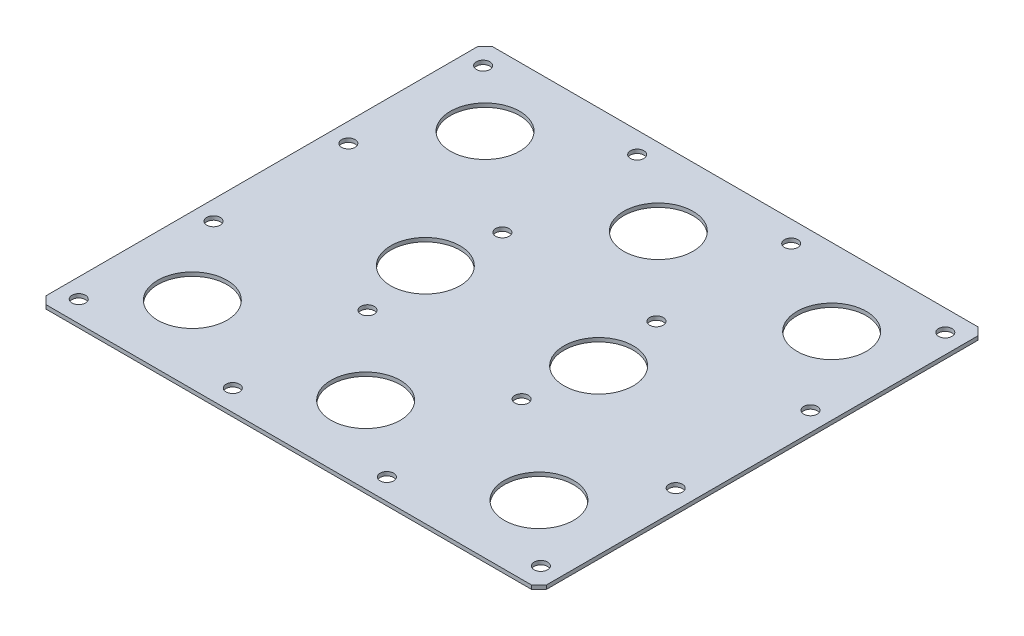
from build123d import *

# Parameters (mm, degrees)
SKETCH1_W                  = 130
SKETCH1_H                  = 116
BOSS_EXTRUDE1_DEPTH        = 1
SKETCH2_R                  = 9
CUT_EXTRUDE1_DEPTH         = 88.120606058
LPATTERN1_COUNT            = 3
LPATTERN1_PITCH            = 38
LPATTERN1_COUNT_DIR2       = 5
LPATTERN1_PITCH_DIR2       = 22.5
CHAMFER1_SIZE              = 2
F_3_5_3_5_DIAMETER_HOLE1_D = 3.5
LPATTERN2_COUNT            = 4
LPATTERN2_PITCH            = 40
LPATTERN2_COUNT_DIR2       = 4
LPATTERN2_PITCH_DIR2       = 35


with BuildPart() as part:
    # Sketch1 → Boss-Extrude1 (new body)
    with BuildSketch(Plane(origin=(0, 0, 0), x_dir=(1, 0, 0), z_dir=(0, 1, 0))):
        Rectangle(SKETCH1_W, SKETCH1_H)
    extrude(amount=BOSS_EXTRUDE1_DEPTH)

    # Sketch2 → Cut-Extrude1 (cut, through all)
    with BuildSketch(Plane(origin=(0, 1, 0), x_dir=(1, 0, 0), z_dir=(0, 1, 0))):
        with Locations(Location((45, -38, 0), (0, 0, 270))):
            Circle(SKETCH2_R)
    cut_extrude1 = extrude(amount=-CUT_EXTRUDE1_DEPTH, mode=Mode.SUBTRACT)

    # LPattern1: Cut-Extrude1 3 × 5, 7 skipped
    with Locations(*[(-j * LPATTERN1_PITCH_DIR2, 0, -i * LPATTERN1_PITCH) for i in range(LPATTERN1_COUNT) for j in range(LPATTERN1_COUNT_DIR2) if (i, j) not in ((0, 0), (0, 1), (0, 3), (1, 0), (1, 2), (1, 4), (2, 1), (2, 3))]):
        add(cut_extrude1, mode=Mode.SUBTRACT)

    # Chamfer1
    chamfer1_edges = [part.edges().sort_by_distance(p)[0] for p in [
        (65, 0.5, 58),
        (-65, 0.5, 58),
        (-65, 0.5, -58),
        (65, 0.5, -58),
    ]]
    chamfer(chamfer1_edges, length=CHAMFER1_SIZE)

    # Ø3.5 (3.5) Diameter Hole1 (through all)
    with Locations(Plane(origin=(0, 1, 0), x_dir=(1, 0, 0), z_dir=(0, 1, 0))):
        with Locations((60, -52.5)):
            f_3_5_3_5_diameter_hole1 = Hole(F_3_5_3_5_DIAMETER_HOLE1_D / 2)

    # LPattern2: 3.5 _3.5_ Diameter Hole1 4 × 4
    with Locations(*[(-i * LPATTERN2_PITCH, 0, -j * LPATTERN2_PITCH_DIR2) for i in range(LPATTERN2_COUNT) for j in range(LPATTERN2_COUNT_DIR2) if (i, j) != (0, 0)]):
        add(f_3_5_3_5_diameter_hole1, mode=Mode.SUBTRACT)


solid = part.part
